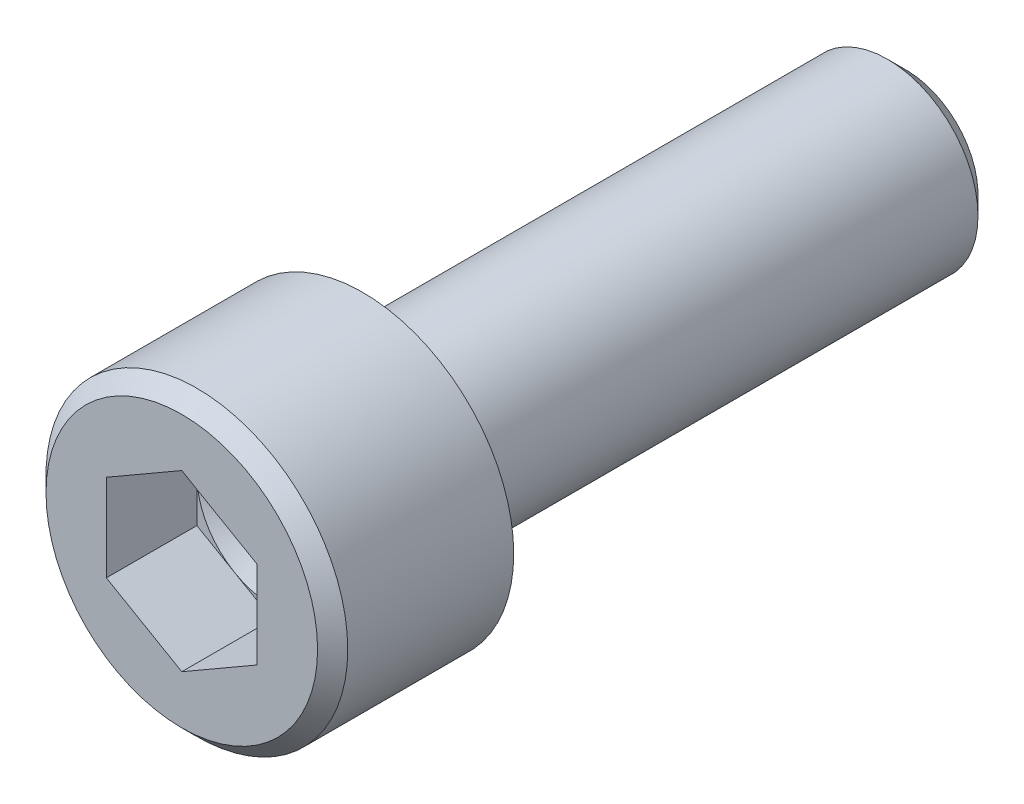
SolidWorks part; units mm, degrees
material "SUS304/0Cr18Ni9"
ref_plane "前视基准面" through (0, 0, 0) normal (0, 0, 1) x (1, 0, 0)
ref_plane "上视基准面" through (0, 0, 0) normal (0, 1, 0) x (1, 0, 0)
ref_plane "右视基准面" through (0, 0, 0) normal (1, 0, 0) x (0, 0, -1)
sketch "草图1" plane through (0, 0, 0) normal (0, 1, 0) x (1, 0, 0)
  line L0 (5, 0) -> (0, 0)
  line L1 (0, 0) -> (0, -6)
  line L2 (0, -6) -> (5, -6)
  line L3 (5, -6) -> (5, 0)
  line L4 (0, 0) -> (0, -6) construction
revolve "旋转1" add sketch "草图1" angle 360 about L4
sketch "草图2" plane through (0, 0, 0) normal (0, 0, -1) x (-1, 0, 0)
  circle A0 centre (0, 0) radius 3
extrude "凸台-拉伸1" add sketch "草图2" along normal blind 18
sketch "草图3" plane through (0, 0, 6) normal (0, 0, 1) x (1, 0, 0)
  line L0 (2.5, 1.4434) -> (0, 2.8868)
  line L1 (0, 2.8868) -> (-2.5, 1.4434)
  line L2 (-2.5, 1.4434) -> (-2.5, -1.4434)
  line L3 (-2.5, -1.4434) -> (0, -2.8868)
  line L4 (0, -2.8868) -> (2.5, -1.4434)
  line L5 (2.5, -1.4434) -> (2.5, 1.4434)
extrude "切除-拉伸1" cut sketch "草图3" against normal blind 3
ref_plane "基准面1" through (0, 0, 0) normal (0, -1, 0) x (1, 0, 0)
sketch "草图4" plane through (0, 0, 0) normal (0, -1, 0) x (1, 0, 0)
  line L0 (2.5, 3) -> (0, 3)
  line L1 (0, 3) -> (0, 1.5566)
  line L2 (0, 1.5566) -> (2.5, 3)
  line L3 (0, 3) -> (0, 1.5566) construction
revolve "切除-旋转1" cut sketch "草图4" angle 360 about L3
chamfer "倒角1" distance 0.5 angle 45 1 edges at (5, 0, 6)
chamfer "倒角2" distance 0.6135 angle 45 1 edges at (-3, 0, -18)
